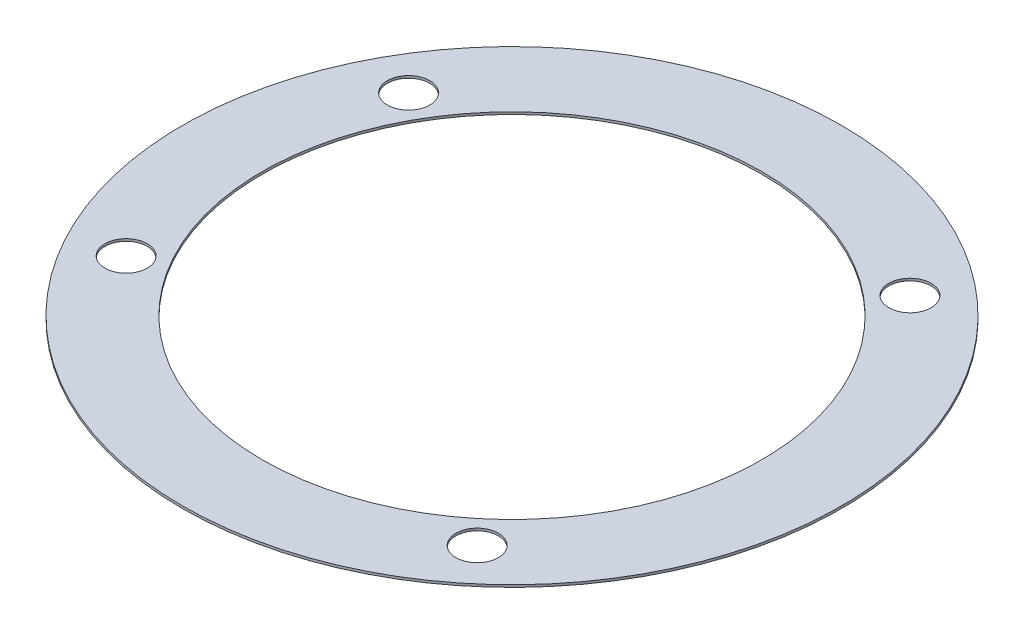
from build123d import *

# Parameters (mm, degrees)
SKETCH1_R                      = 111.125
SKETCH1_R_2                    = 84.2
BOSS_EXTRUDE1_DEPTH            = 0.79375
F_9_16_0_5625_DIAMETER_HOLE1_D = 14.2875
F_9_16_0_5625_DIAMETER_HOLE2_D = 14.2875


with BuildPart() as part:
    # Sketch1 → Boss-Extrude1 (new body)
    with BuildSketch(Plane(origin=(0, 0, 0), x_dir=(1, 0, 0), z_dir=(0, 1, 0))):
        with Locations(Location((0, 0, 0), (0, 0, 270))):
            Circle(SKETCH1_R)
        with Locations(Location((0, 0, 0), (0, 0, 270))):
            Circle(SKETCH1_R_2, mode=Mode.SUBTRACT)
    extrude(amount=BOSS_EXTRUDE1_DEPTH)

    # 9/16 (0.5625) Diameter Hole1 (through all)
    with Locations(Plane(origin=(61.2154, 0.79375, -72.9742), x_dir=(0, 0, 1), z_dir=(0, 1, 0))):
        with Locations((0, 0)):
            f_9_16_0_5625_diameter_hole1 = Hole(F_9_16_0_5625_DIAMETER_HOLE1_D / 2)

    # 9/16 (0.5625) Diameter Hole2 (through all)
    with Locations(Plane(origin=(0, 0, 0), x_dir=(-1, 0, 0), z_dir=(0, -1, 0))):
        with Locations((82.4992, 47.625)):
            f_9_16_0_5625_diameter_hole2 = Hole(F_9_16_0_5625_DIAMETER_HOLE2_D / 2)

    # Mirror1: 9/16 (0.5625) Diameter Hole1, 9/16 (0.5625) Diameter Hole2 across plane
    add(f_9_16_0_5625_diameter_hole1.mirror(Plane.XY), mode=Mode.SUBTRACT)
    add(f_9_16_0_5625_diameter_hole2.mirror(Plane.XY), mode=Mode.SUBTRACT)


solid = part.part
